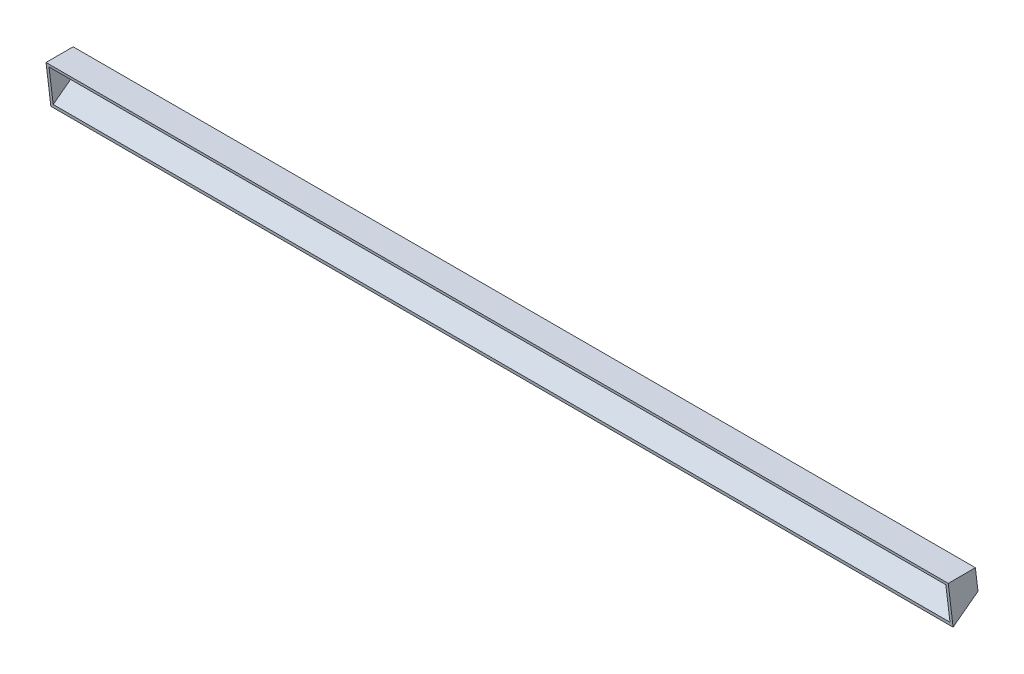
SolidWorks part; units mm, degrees
ref_plane "Front plane" through (0, 0, 0) normal (0, 0, 1) x (1, 0, 0)
ref_plane "Top plane" through (0, 0, 0) normal (0, 1, 0) x (1, 0, 0)
ref_plane "Right plane" through (0, 0, 0) normal (1, 0, 0) x (0, 0, -1)
sketch "Sketch1" plane through (0, 0, 0) normal (1, 0, 0) x (0, 0, -1)
  line L0 (0, 0) -> (-20, 0)
  line L3 (-20, 0) -> (-16.4142, -29.7849)
  line L5 (-16.4142, -29.7849) -> (1.9298, -16.0295)
  line L9 (1.9298, -16.0295) -> (0, 0)
  dimension "D3" = 30
  dimension "D1" = 20
  dimension "D2" = 120
  dimension "D4" = 96.865
extrude "Boss-Extrude1" add sketch "Sketch1" along normal blind 2
sketch "Sketch2" plane through (0, 0, 0) normal (-1, 0, 0) x (0, 0, 1)
  line L0 (0, 0) -> (20, 0) construction
  line L1 (-1.9298, -16.0295) -> (0, 0) construction
  line L2 (16.4142, -29.7849) -> (-1.9298, -16.0295) construction
  line L3 (0, 0) -> (20, 0)
  line L4 (-1.9298, -16.0295) -> (0, 0)
  line L5 (16.4142, -29.7849) -> (-1.9298, -16.0295)
  line L6 (16.6903, -27.4921) -> (0.1939, -15.1222)
  line L7 (0.1939, -15.1222) -> (1.7737, -2)
  line L8 (1.7737, -2) -> (19.7592, -2)
  line L9 (20, 0) -> (16.4142, -29.7849) construction
  line L10 (20, 0) -> (19.7592, -2)
  line L11 (16.6903, -27.4921) -> (16.4142, -29.7849)
  line L12 (17.6141, -28.1848) -> (0.1939, -15.1222) construction
  line L14 (1.7737, -2) -> (20, -2) construction
  dimension "D1" = 2
extrude "Boss-Extrude2" add sketch "Sketch2" along normal blind 661
sketch "Sketch3" plane through (-661, 0, 0) normal (-1, 0, 0) x (0, 0, 1)
  line L4 (20, 0) -> (0, 0)
  line L5 (16.4142, -29.7849) -> (20, 0)
  line L6 (-1.9298, -16.0295) -> (16.4142, -29.7849)
  line L7 (0, 0) -> (-1.9298, -16.0295)
  line L8 (20, 0) -> (0, 0)
  line L9 (16.4142, -29.7849) -> (20, 0)
  line L10 (-1.9298, -16.0295) -> (16.4142, -29.7849)
  line L11 (0, 0) -> (-1.9298, -16.0295)
  dimension "D1" = 0
extrude "Boss-Extrude3" add sketch "Sketch3" along normal blind 2
